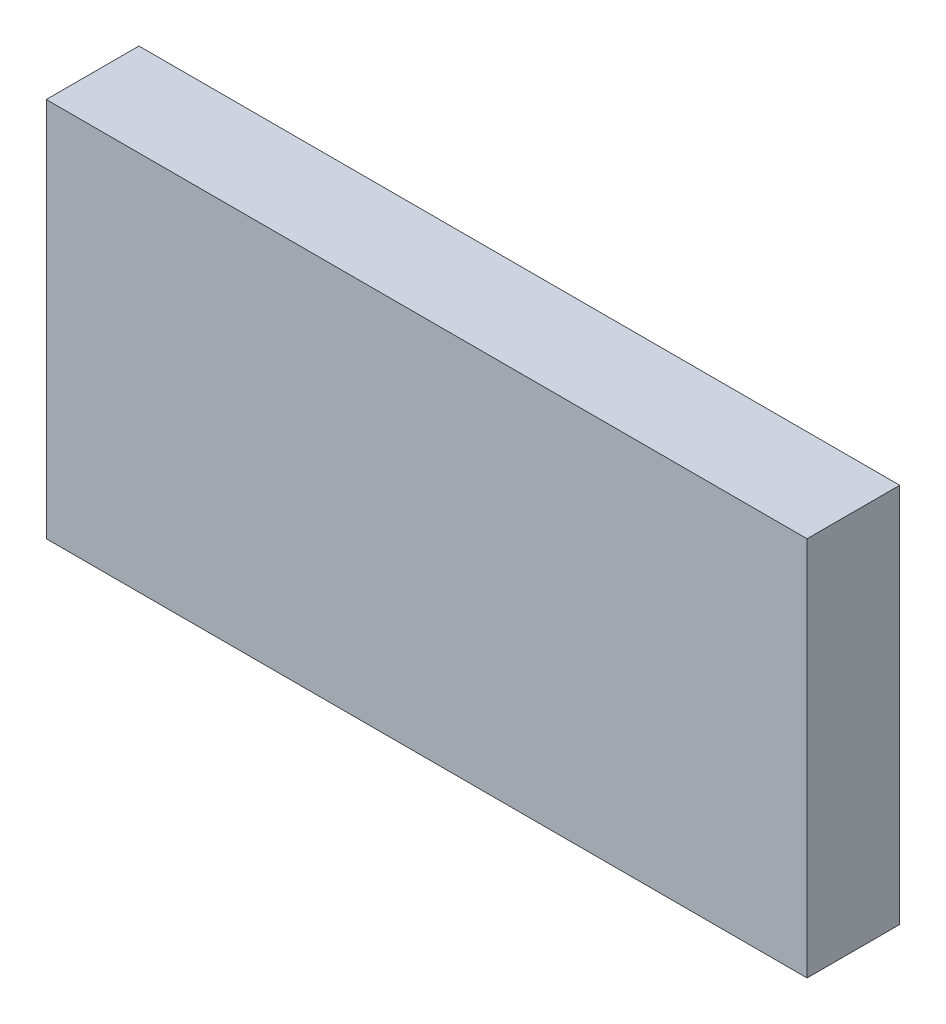
from build123d import *

# Parameters (mm, degrees)
SKETCH1_W           = 390
SKETCH1_H           = 47.5
BOSS_EXTRUDE1_DEPTH = 195
SHELL1_T            = -6


with BuildPart() as part:
    # Sketch1 → Boss-Extrude1 (new body)
    with BuildSketch(Plane(origin=(0, 0, 0), x_dir=(1, 0, 0), z_dir=(0, 1, 0))):
        Rectangle(SKETCH1_W, SKETCH1_H)
    extrude(amount=BOSS_EXTRUDE1_DEPTH)

    # Shell1
    shell1_openings = [part.faces().sort_by_distance(p)[0] for p in [
        (0, 97.5, -23.75),
    ]]
    offset(amount=SHELL1_T, openings=shell1_openings, kind=Kind.INTERSECTION)


solid = part.part
